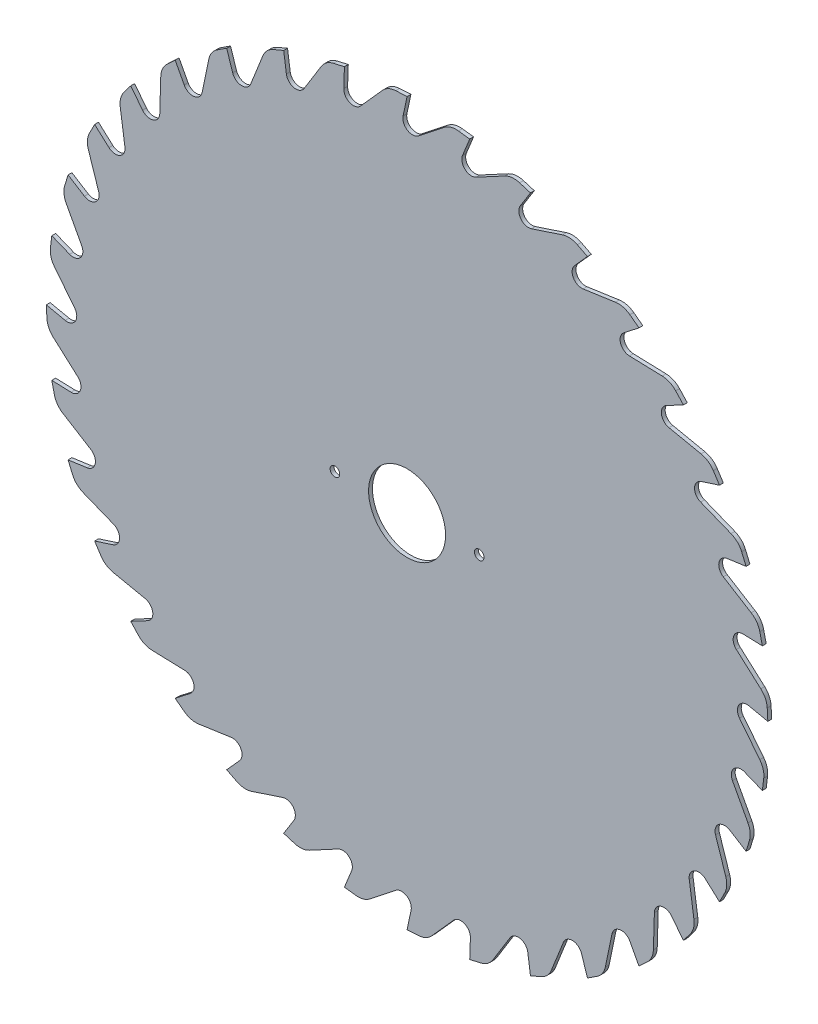
from build123d import *

# Parameters (mm, degrees)
DICKE_DEPTH               = 4
SKETCH2_R                 = 5
SKETCH2_R_2               = 40
LINEAR_CUT_EXTRUDE1_DEPTH = 531.34517062


with BuildPart() as part:
    # Sketch1 → Dicke (new body)
    with BuildSketch(Plane.XY):
        with BuildLine():
            Line((0, 375), (-4.158233816, 355.437047985))
            ThreePointArc((-4.158233816, 355.437047985), (0.342498495, 344.8659498), (11.814061112, 345.504666719))
            Line((11.814061112, 345.504666719), (38.57216905, 366.598391999))
            ThreePointArc((38.57216905, 366.598391999), (45.567153672, 370.152807368), (53.391193761, 370.742786315))
            Line((53.391193761, 370.742786315), (65.118066625, 369.30290738))
            Line((65.118066625, 369.30290738), (57.625934757, 350.759230288))
            ThreePointArc((57.625934757, 350.759230288), (60.222638895, 339.567186873), (71.630834729, 338.204184304))
            Line((71.630834729, 338.204184304), (101.645313837, 354.330951818))
            ThreePointArc((101.645313837, 354.330951818), (109.151246677, 356.616701298), (116.958870785, 355.839086836))
            Line((116.958870785, 355.839086836), (128.257553747, 352.384732795))
            Line((128.257553747, 352.384732795), (117.659168462, 335.423770872))
            ThreePointArc((117.659168462, 335.423770872), (118.272944887, 323.950846803), (129.27114168, 320.627538888))
            Line((129.27114168, 320.627538888), (161.630017199, 331.297344966))
            ThreePointArc((161.630017199, 331.297344966), (169.418834284, 332.244977217), (176.972811705, 330.123396767))
            Line((176.972811705, 330.123396767), (187.5, 324.759526419))
            Line((187.5, 324.759526419), (174.117387873, 309.89662991))
            ThreePointArc((174.117387873, 309.89662991), (172.729587297, 298.491424179), (182.983610405, 293.308787948))
            Line((182.983610405, 293.308787948), (216.703674276, 298.197435932))
            ThreePointArc((216.703674276, 298.197435932), (224.538716342, 297.778157627), (231.609523293, 294.377074338))
            Line((231.609523293, 294.377074338), (241.045353632, 287.26666617))
            Line((241.045353632, 287.26666617), (225.28513856, 274.953436663))
            ThreePointArc((225.28513856, 274.953436663), (221.937928603, 263.962490676), (231.136214722, 257.077997908))
            Line((231.136214722, 257.077997908), (265.192899868, 256.036948703))
            ThreePointArc((265.192899868, 256.036948703), (272.836103126, 254.2634994), (279.208896716, 249.686253467))
            Line((279.208896716, 249.686253467), (287.26666617, 241.045353632))
            Line((287.26666617, 241.045353632), (269.607714312, 231.655922377))
            ThreePointArc((269.607714312, 231.655922377), (264.402798254, 221.413190465), (272.265862115, 213.03602299))
            Line((272.265862115, 213.03602299), (305.624373391, 206.096908348))
            ThreePointArc((305.624373391, 206.096908348), (312.843502978, 203.023173408), (318.324649099, 197.408842132))
            Line((318.324649099, 197.408842132), (324.759526419, 187.5))
            Line((324.759526419, 187.5), (305.738396093, 181.319660112))
            ThreePointArc((305.738396093, 181.319660112), (298.833922674, 172.136362502), (305.122849061, 162.521056314))
            Line((305.122849061, 162.521056314), (336.769604982, 149.894717723))
            ThreePointArc((336.769604982, 149.894717723), (343.345311299, 145.614091026), (347.768268099, 139.133263022))
            Line((347.768268099, 139.133263022), (352.384732795, 128.257553747))
            Line((352.384732795, 128.257553747), (332.57937142, 125.474091728))
            ThreePointArc((332.57937142, 125.474091728), (324.185129571, 117.62925827), (328.708832638, 107.067969582))
            Line((328.708832638, 107.067969582), (357.68226254, 89.13805195))
            ThreePointArc((357.68226254, 89.13805195), (363.414746077, 83.780598173), (366.645124252, 76.63019012))
            Line((366.645124252, 76.63019012), (369.30290738, 65.118066625))
            Line((369.30290738, 65.118066625), (349.315090839, 65.816056559))
            ThreePointArc((349.315090839, 65.816056559), (339.686135352, 59.548048549), (342.30716467, 48.361676773))
            Line((342.30716467, 48.361676773), (367.726925546, 25.672971575))
            ThreePointArc((367.726925546, 25.672971575), (372.442007692, 19.401474239), (374.381653836, 11.798747668))
            Line((374.381653836, 11.798747668), (375, 0))
            Line((375, 0), (355.437047985, 4.158233816))
            ThreePointArc((355.437047985, 4.158233816), (344.8659498, -0.342498495), (345.504666719, -11.814061112))
            Line((345.504666719, -11.814061112), (366.598391999, -38.57216905))
            ThreePointArc((366.598391999, -38.57216905), (370.152807368, -45.567153672), (370.742786315, -53.391193761))
            Line((370.742786315, -53.391193761), (369.30290738, -65.118066625))
            Line((369.30290738, -65.118066625), (350.759230288, -57.625934757))
            ThreePointArc((350.759230288, -57.625934757), (339.567186873, -60.222638895), (338.204184304, -71.630834729))
            Line((338.204184304, -71.630834729), (354.330951818, -101.645313837))
            ThreePointArc((354.330951818, -101.645313837), (356.616701298, -109.151246677), (355.839086836, -116.958870785))
            Line((355.839086836, -116.958870785), (352.384732795, -128.257553747))
            Line((352.384732795, -128.257553747), (335.423770872, -117.659168462))
            ThreePointArc((335.423770872, -117.659168462), (323.950846803, -118.272944887), (320.627538888, -129.27114168))
            Line((320.627538888, -129.27114168), (331.297344966, -161.630017199))
            ThreePointArc((331.297344966, -161.630017199), (332.244977217, -169.418834284), (330.123396767, -176.972811705))
            Line((330.123396767, -176.972811705), (324.759526419, -187.5))
            Line((324.759526419, -187.5), (309.89662991, -174.117387873))
            ThreePointArc((309.89662991, -174.117387873), (298.491424179, -172.729587297), (293.308787948, -182.983610405))
            Line((293.308787948, -182.983610405), (298.197435932, -216.703674276))
            ThreePointArc((298.197435932, -216.703674276), (297.778157627, -224.538716342), (294.377074338, -231.609523293))
            Line((294.377074338, -231.609523293), (287.26666617, -241.045353632))
            Line((287.26666617, -241.045353632), (274.953436663, -225.28513856))
            ThreePointArc((274.953436663, -225.28513856), (263.962490676, -221.937928603), (257.077997908, -231.136214722))
            Line((257.077997908, -231.136214722), (256.036948703, -265.192899868))
            ThreePointArc((256.036948703, -265.192899868), (254.2634994, -272.836103126), (249.686253467, -279.208896716))
            Line((249.686253467, -279.208896716), (241.045353632, -287.26666617))
            Line((241.045353632, -287.26666617), (231.655922377, -269.607714312))
            ThreePointArc((231.655922377, -269.607714312), (221.413190465, -264.402798254), (213.03602299, -272.265862115))
            Line((213.03602299, -272.265862115), (206.096908348, -305.624373391))
            ThreePointArc((206.096908348, -305.624373391), (203.023173408, -312.843502978), (197.408842132, -318.324649099))
            Line((197.408842132, -318.324649099), (187.5, -324.759526419))
            Line((187.5, -324.759526419), (181.319660113, -305.738396093))
            ThreePointArc((181.319660113, -305.738396093), (172.136362502, -298.833922674), (162.521056314, -305.122849061))
            Line((162.521056314, -305.122849061), (149.894717723, -336.769604983))
            ThreePointArc((149.894717723, -336.769604983), (145.614091026, -343.345311299), (139.133263022, -347.768268099))
            Line((139.133263022, -347.768268099), (128.257553747, -352.384732795))
            Line((128.257553747, -352.384732795), (125.474091728, -332.57937142))
            ThreePointArc((125.474091728, -332.57937142), (117.62925827, -324.185129571), (107.067969582, -328.708832638))
            Line((107.067969582, -328.708832638), (89.13805195, -357.68226254))
            ThreePointArc((89.13805195, -357.68226254), (83.780598173, -363.414746077), (76.63019012, -366.645124252))
            Line((76.63019012, -366.645124252), (65.118066625, -369.30290738))
            Line((65.118066625, -369.30290738), (65.816056559, -349.315090839))
            ThreePointArc((65.816056559, -349.315090839), (59.548048549, -339.686135352), (48.361676773, -342.30716467))
            Line((48.361676773, -342.30716467), (25.672971575, -367.726925546))
            ThreePointArc((25.672971575, -367.726925546), (19.401474239, -372.442007692), (11.798747668, -374.381653836))
            Line((11.798747668, -374.381653836), (0, -375))
            Line((0, -375), (4.158233816, -355.437047985))
            ThreePointArc((4.158233816, -355.437047985), (-0.342498495, -344.8659498), (-11.814061112, -345.504666719))
            Line((-11.814061112, -345.504666719), (-38.57216905, -366.598391999))
            ThreePointArc((-38.57216905, -366.598391999), (-45.567153672, -370.152807368), (-53.391193761, -370.742786315))
            Line((-53.391193761, -370.742786315), (-65.118066625, -369.30290738))
            Line((-65.118066625, -369.30290738), (-57.625934757, -350.759230288))
            ThreePointArc((-57.625934757, -350.759230288), (-60.222638895, -339.567186873), (-71.630834729, -338.204184304))
            Line((-71.630834729, -338.204184304), (-101.645313837, -354.330951818))
            ThreePointArc((-101.645313837, -354.330951818), (-109.151246677, -356.616701299), (-116.958870785, -355.839086836))
            Line((-116.958870785, -355.839086836), (-128.257553747, -352.384732795))
            Line((-128.257553747, -352.384732795), (-117.659168462, -335.423770872))
            ThreePointArc((-117.659168462, -335.423770872), (-118.272944887, -323.950846803), (-129.27114168, -320.627538888))
            Line((-129.27114168, -320.627538888), (-161.630017199, -331.297344966))
            ThreePointArc((-161.630017199, -331.297344966), (-169.418834284, -332.244977217), (-176.972811705, -330.123396767))
            Line((-176.972811705, -330.123396767), (-187.5, -324.759526419))
            Line((-187.5, -324.759526419), (-174.117387873, -309.89662991))
            ThreePointArc((-174.117387873, -309.89662991), (-172.729587297, -298.491424179), (-182.983610405, -293.308787948))
            Line((-182.983610405, -293.308787948), (-216.703674276, -298.197435932))
            ThreePointArc((-216.703674276, -298.197435932), (-224.538716342, -297.778157627), (-231.609523293, -294.377074338))
            Line((-231.609523293, -294.377074338), (-241.045353632, -287.26666617))
            Line((-241.045353632, -287.26666617), (-225.28513856, -274.953436663))
            ThreePointArc((-225.28513856, -274.953436663), (-221.937928603, -263.962490676), (-231.136214722, -257.077997908))
            Line((-231.136214722, -257.077997908), (-265.192899868, -256.036948703))
            ThreePointArc((-265.192899868, -256.036948703), (-272.836103126, -254.2634994), (-279.208896716, -249.686253467))
            Line((-279.208896716, -249.686253467), (-287.26666617, -241.045353632))
            Line((-287.26666617, -241.045353632), (-269.607714312, -231.655922377))
            ThreePointArc((-269.607714312, -231.655922377), (-264.402798254, -221.413190465), (-272.265862115, -213.03602299))
            Line((-272.265862115, -213.03602299), (-305.624373391, -206.096908348))
            ThreePointArc((-305.624373391, -206.096908348), (-312.843502978, -203.023173408), (-318.324649099, -197.408842132))
            Line((-318.324649099, -197.408842132), (-324.759526419, -187.5))
            Line((-324.759526419, -187.5), (-305.738396093, -181.319660113))
            ThreePointArc((-305.738396093, -181.319660113), (-298.833922674, -172.136362502), (-305.122849061, -162.521056314))
            Line((-305.122849061, -162.521056314), (-336.769604982, -149.894717723))
            ThreePointArc((-336.769604982, -149.894717723), (-343.345311299, -145.614091026), (-347.768268099, -139.133263022))
            Line((-347.768268099, -139.133263022), (-352.384732795, -128.257553747))
            Line((-352.384732795, -128.257553747), (-332.57937142, -125.474091728))
            ThreePointArc((-332.57937142, -125.474091728), (-324.185129571, -117.62925827), (-328.708832638, -107.067969582))
            Line((-328.708832638, -107.067969582), (-357.68226254, -89.13805195))
            ThreePointArc((-357.68226254, -89.13805195), (-363.414746077, -83.780598173), (-366.645124252, -76.63019012))
            Line((-366.645124252, -76.63019012), (-369.30290738, -65.118066625))
            Line((-369.30290738, -65.118066625), (-349.315090839, -65.816056559))
            ThreePointArc((-349.315090839, -65.816056559), (-339.686135352, -59.548048549), (-342.30716467, -48.361676773))
            Line((-342.30716467, -48.361676773), (-367.726925546, -25.672971575))
            ThreePointArc((-367.726925546, -25.672971575), (-372.442007692, -19.401474239), (-374.381653836, -11.798747668))
            Line((-374.381653836, -11.798747668), (-375, 0))
            Line((-375, 0), (-355.437047985, -4.158233816))
            ThreePointArc((-355.437047985, -4.158233816), (-344.8659498, 0.342498495), (-345.504666719, 11.814061112))
            Line((-345.504666719, 11.814061112), (-366.598391999, 38.57216905))
            ThreePointArc((-366.598391999, 38.57216905), (-370.152807368, 45.567153672), (-370.742786315, 53.391193761))
            Line((-370.742786315, 53.391193761), (-369.30290738, 65.118066625))
            Line((-369.30290738, 65.118066625), (-350.759230288, 57.625934757))
            ThreePointArc((-350.759230288, 57.625934757), (-339.567186873, 60.222638895), (-338.204184304, 71.630834729))
            Line((-338.204184304, 71.630834729), (-354.330951818, 101.645313837))
            ThreePointArc((-354.330951818, 101.645313837), (-356.616701299, 109.151246677), (-355.839086836, 116.958870785))
            Line((-355.839086836, 116.958870785), (-352.384732795, 128.257553747))
            Line((-352.384732795, 128.257553747), (-335.423770872, 117.659168462))
            ThreePointArc((-335.423770872, 117.659168462), (-323.950846803, 118.272944887), (-320.627538888, 129.27114168))
            Line((-320.627538888, 129.27114168), (-331.297344966, 161.630017199))
            ThreePointArc((-331.297344966, 161.630017199), (-332.244977217, 169.418834284), (-330.123396767, 176.972811705))
            Line((-330.123396767, 176.972811705), (-324.759526419, 187.5))
            Line((-324.759526419, 187.5), (-309.89662991, 174.117387873))
            ThreePointArc((-309.89662991, 174.117387873), (-298.491424179, 172.729587297), (-293.308787948, 182.983610405))
            Line((-293.308787948, 182.983610405), (-298.197435932, 216.703674276))
            ThreePointArc((-298.197435932, 216.703674276), (-297.778157627, 224.538716342), (-294.377074338, 231.609523293))
            Line((-294.377074338, 231.609523293), (-287.26666617, 241.045353632))
            Line((-287.26666617, 241.045353632), (-274.953436663, 225.28513856))
            ThreePointArc((-274.953436663, 225.28513856), (-263.962490676, 221.937928603), (-257.077997908, 231.136214722))
            Line((-257.077997908, 231.136214722), (-256.036948703, 265.192899868))
            ThreePointArc((-256.036948703, 265.192899868), (-254.2634994, 272.836103126), (-249.686253467, 279.208896716))
            Line((-249.686253467, 279.208896716), (-241.045353632, 287.26666617))
            Line((-241.045353632, 287.26666617), (-231.655922377, 269.607714312))
            ThreePointArc((-231.655922377, 269.607714312), (-221.413190465, 264.402798254), (-213.03602299, 272.265862115))
            Line((-213.03602299, 272.265862115), (-206.096908348, 305.624373391))
            ThreePointArc((-206.096908348, 305.624373391), (-203.023173408, 312.843502978), (-197.408842132, 318.324649099))
            Line((-197.408842132, 318.324649099), (-187.5, 324.759526419))
            Line((-187.5, 324.759526419), (-181.319660113, 305.738396093))
            ThreePointArc((-181.319660113, 305.738396093), (-172.136362502, 298.833922674), (-162.521056314, 305.122849061))
            Line((-162.521056314, 305.122849061), (-149.894717723, 336.769604982))
            ThreePointArc((-149.894717723, 336.769604982), (-145.614091026, 343.345311299), (-139.133263022, 347.768268099))
            Line((-139.133263022, 347.768268099), (-128.257553747, 352.384732795))
            Line((-128.257553747, 352.384732795), (-125.474091728, 332.57937142))
            ThreePointArc((-125.474091728, 332.57937142), (-117.62925827, 324.185129571), (-107.067969582, 328.708832638))
            Line((-107.067969582, 328.708832638), (-89.13805195, 357.68226254))
            ThreePointArc((-89.13805195, 357.68226254), (-83.780598173, 363.414746077), (-76.63019012, 366.645124252))
            Line((-76.63019012, 366.645124252), (-65.118066625, 369.30290738))
            Line((-65.118066625, 369.30290738), (-65.816056559, 349.315090839))
            ThreePointArc((-65.816056559, 349.315090839), (-59.548048549, 339.686135352), (-48.361676773, 342.30716467))
            Line((-48.361676773, 342.30716467), (-25.672971575, 367.726925546))
            ThreePointArc((-25.672971575, 367.726925546), (-19.401474239, 372.442007692), (-11.798747668, 374.381653836))
            Line((-11.798747668, 374.381653836), (0, 375))
        make_face()
    extrude(amount=DICKE_DEPTH)

    # Sketch2 → Linear Cut Extrude1 (cut, through all)
    with BuildSketch(Plane.XY.offset(4)):
        with Locations((75, 0)):
            Circle(SKETCH2_R)
        with Locations((-75, 0)):
            Circle(SKETCH2_R)
        Circle(SKETCH2_R_2)
    extrude(amount=-LINEAR_CUT_EXTRUDE1_DEPTH, mode=Mode.SUBTRACT)


solid = part.part
